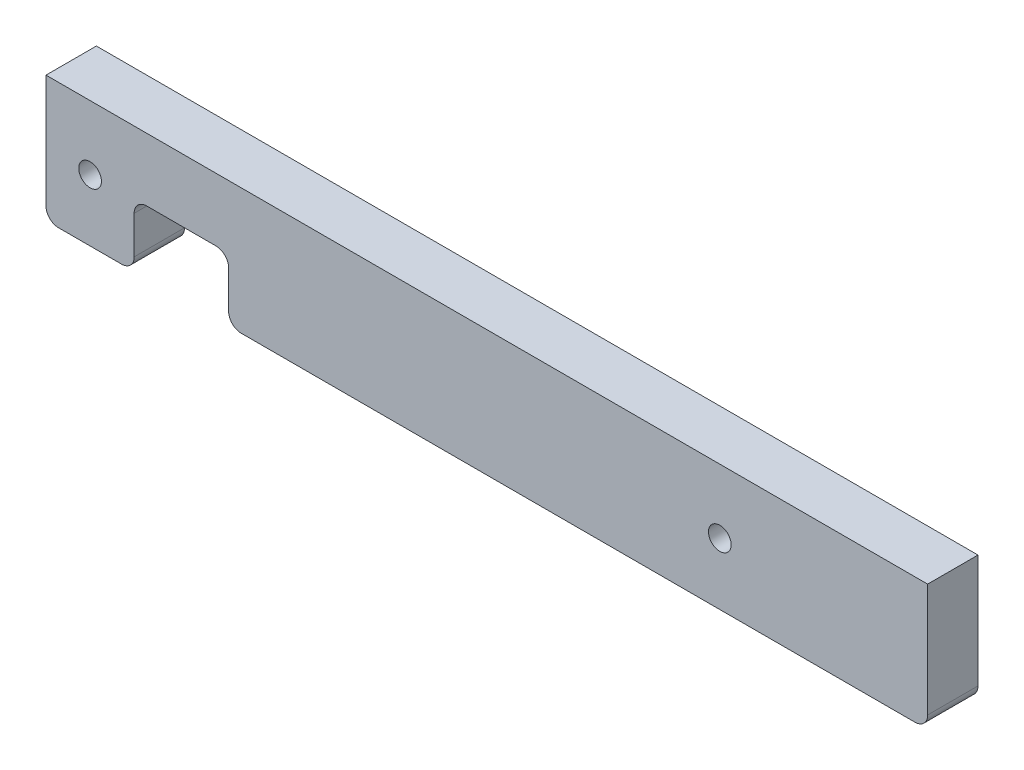
SolidWorks part; units mm, degrees
material "Q235B"
ref_plane "Front Plane" through (0, 0, 0) normal (0, 0, 1) x (1, 0, 0)
ref_plane "Top Plane" through (0, 0, 0) normal (0, 1, 0) x (1, 0, 0)
ref_plane "Right Plane" through (0, 0, 0) normal (1, 0, 0) x (0, 0, -1)
sketch "Sketch1" plane through (0, 0, 0) normal (0, 0, 1) x (1, 0, 0)
  line L0 (70, 0) -> (70, 50)
  line L1 (70, 50) -> (145, 50)
  line L2 (0, 0) -> (0, 100)
  line L3 (0, 100) -> (700, 100)
  line L4 (700, 0) -> (700, 100)
  line L5 (700, 0) -> (145, 0)
  line L6 (145, 50) -> (145, 0)
  line L7 (70, 0) -> (0, 0)
  circle A0 centre (35, 49) radius 9
  circle A1 centre (535, 49) radius 9
  dimension "D3" = 18
  dimension "D4" = 51
  dimension "D5" = 165
  dimension "D6" = 500
  dimension "D1" = 700
  dimension "D2" = 100
  dimension "D7" = 75
  dimension "D8" = 50
  dimension "D9" = 70
extrude "Boss-Extrude1" add sketch "Sketch1" along normal blind 40
fillet "Fillet1" radius 10 6 edges at (700, 0, 20) (0, 0, 20) (70, 0, 20) (145, 0, 20) (70, 50, 20) (145, 50, 20)
